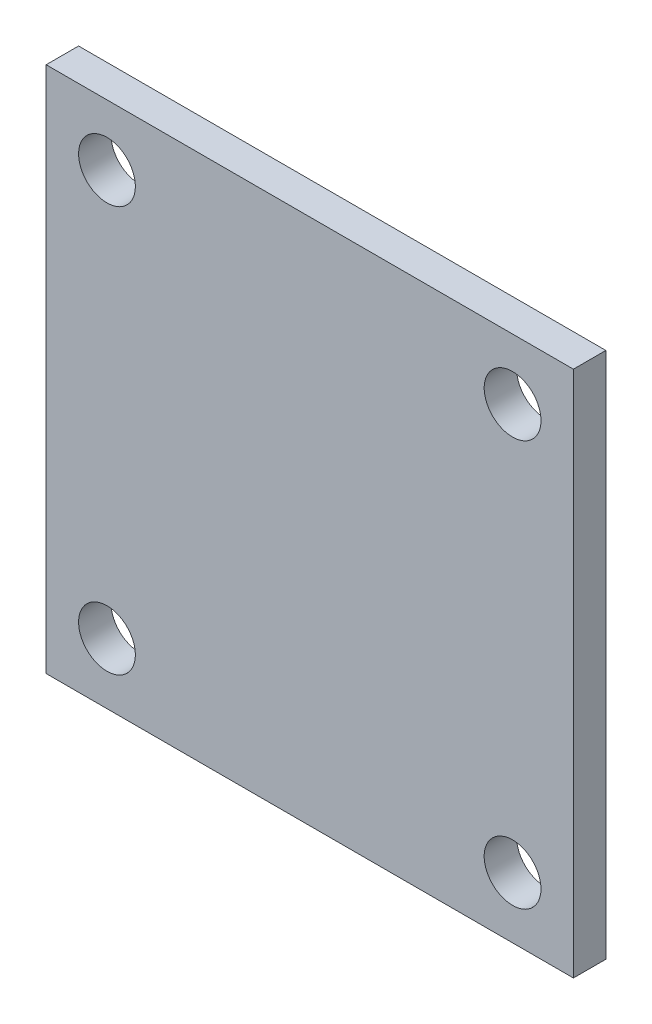
from build123d import *

# Parameters (mm, degrees)
SKETCH1_W           = 130
SKETCH1_H           = 130
SKETCH1_R           = 7
BOSS_EXTRUDE1_DEPTH = 8


with BuildPart() as part:
    # Sketch1 → Boss-Extrude1 (new body)
    with BuildSketch(Plane.XY):
        Rectangle(SKETCH1_W, SKETCH1_H)
        with Locations((-50, 50)):
            Circle(SKETCH1_R, mode=Mode.SUBTRACT)
        with Locations((50, 50)):
            Circle(SKETCH1_R, mode=Mode.SUBTRACT)
        with Locations((50, -50)):
            Circle(SKETCH1_R, mode=Mode.SUBTRACT)
        with Locations((-50, -50)):
            Circle(SKETCH1_R, mode=Mode.SUBTRACT)
    extrude(amount=BOSS_EXTRUDE1_DEPTH)


solid = part.part
